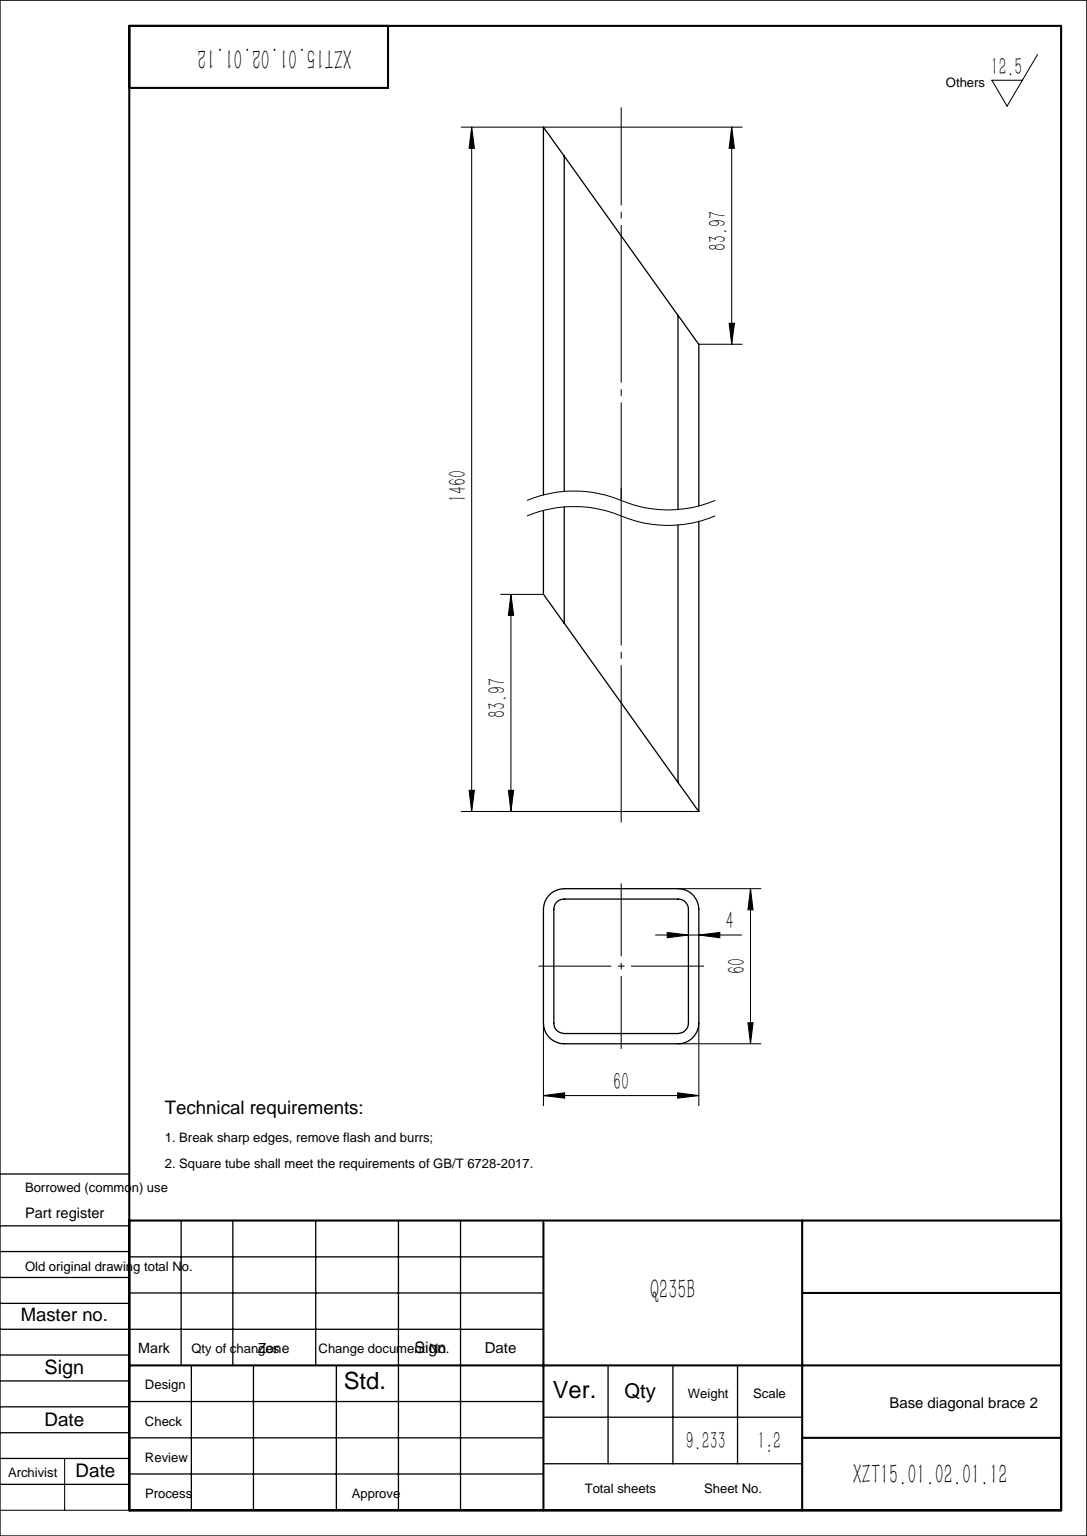
from build123d import *

# Parameters (mm, degrees)
GB_T_6728_2002_SQUARE_HOLLOW_SECTION_60_DEPTH = 1460
CUT_EXTRUDE1_DEPTH                            = 1462.5402834
CUT_EXTRUDE1_DEPTH_BACK                       = 1462.5402834


with BuildPart() as part:
    # Sketch1 → GB/T 6728-2002 square hollow section 60×60×4(1) (new body)
    with BuildSketch(Plane(origin=(0, 0, 0), x_dir=(-1, 0, 0), z_dir=(0, 1, 0))):
        with BuildLine():
            Line((-22, -30), (22, -30))
            ThreePointArc((22, -30), (27.656854249, -27.656854249), (30, -22))
            Line((30, -22), (30, 22))
            ThreePointArc((30, 22), (27.656854249, 27.656854249), (22, 30))
            Line((22, 30), (-22, 30))
            ThreePointArc((-22, 30), (-27.656854249, 27.656854249), (-30, 22))
            Line((-30, 22), (-30, -22))
            ThreePointArc((-30, -22), (-27.656854249, -27.656854249), (-22, -30))
        make_face()
        with BuildLine():
            Line((-22, -26), (22, -26))
            ThreePointArc((22, -26), (24.828427125, -24.828427125), (26, -22))
            Line((26, -22), (26, 22))
            ThreePointArc((26, 22), (24.828427125, 24.828427125), (22, 26))
            Line((22, 26), (-22, 26))
            ThreePointArc((-22, 26), (-24.828427125, 24.828427125), (-26, 22))
            Line((-26, 22), (-26, -22))
            ThreePointArc((-26, -22), (-24.828427125, -24.828427125), (-22, -26))
        make_face(mode=Mode.SUBTRACT)
    extrude(amount=GB_T_6728_2002_SQUARE_HOLLOW_SECTION_60_DEPTH)

    # Sketch2 → Cut-Extrude1 (cut, two sides: drawn at the far end of the back side and taken through both)
    with BuildSketch(Plane.XY.offset(30).offset(-CUT_EXTRUDE1_DEPTH_BACK)):
        Polygon((-30, 1460), (30, 1376.03139841), (30, 1460), align=None)
        Polygon((-30, 0), (-30, 83.96860159), (30, 0), align=None)
    extrude(amount=CUT_EXTRUDE1_DEPTH + CUT_EXTRUDE1_DEPTH_BACK, mode=Mode.SUBTRACT)


solid = part.part
